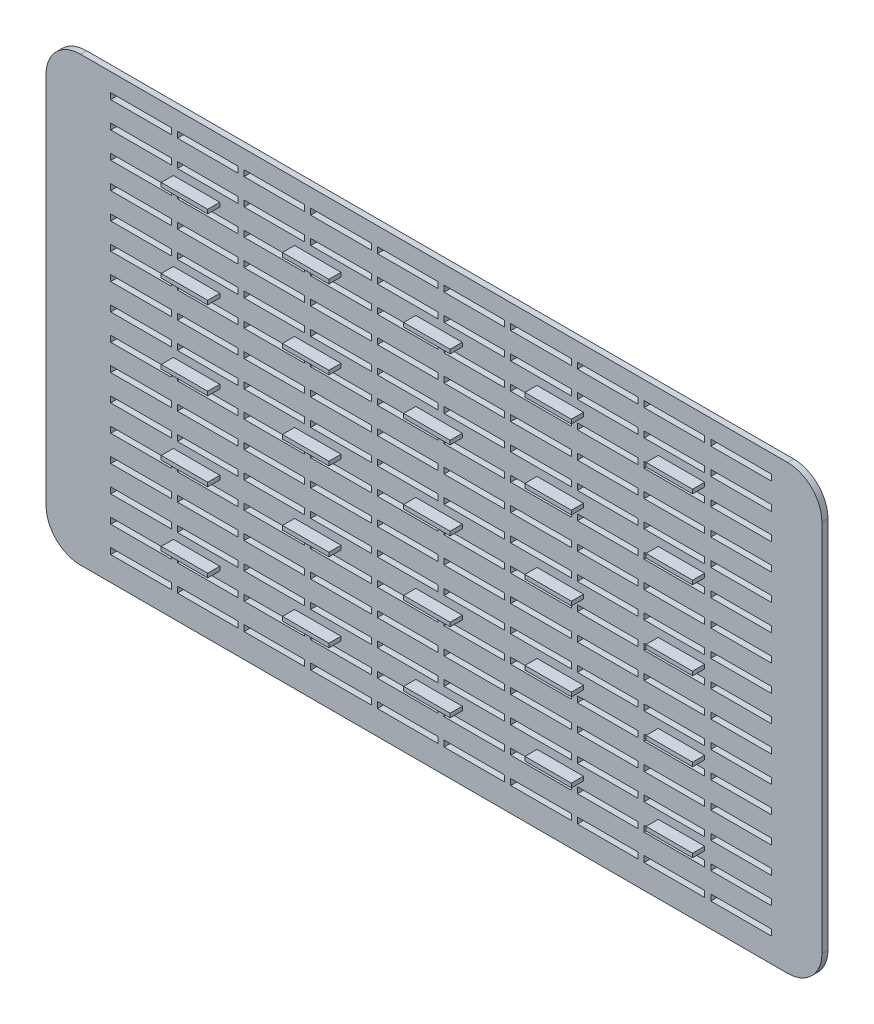
SolidWorks part; units mm, degrees
ref_plane "前视" through (0, 0, 0) normal (0, 0, 1) x (1, 0, 0)
ref_plane "上视" through (0, 0, 0) normal (0, 1, 0) x (1, 0, 0)
ref_plane "右视" through (0, 0, 0) normal (1, 0, 0) x (0, 0, -1)
sketch "草图1" plane through (0, 0, 0) normal (0, 0, 1) x (1, 0, 0)
  line L1 (-192, -109.5) -> (192, -109.5)
  line L2 (-192, -109.5) -> (-192, 109.5)
  line L3 (-192, 109.5) -> (192, 109.5)
  line L4 (192, -109.5) -> (192, 109.5)
  line L5 (-192, -109.5) -> (192, 109.5) construction
  line L6 (-192, 109.5) -> (192, -109.5) construction
  point P0 (0, 0)
  dimension "D1" = 384
  dimension "D2" = 219
extrude "凸台-拉伸1" add sketch "草图1" along normal blind 3
fillet "圆角1" radius 17 4 edges at (-192, -109.5, 1.5) (-192, 109.5, 1.5) (192, -109.5, 1.5) (192, 109.5, 1.5)
sketch "草图2" plane through (0, 0, 3) normal (0, 0, 1) x (1, 0, 0)
  line L0 (175, 109.5) -> (-175, 109.5) construction
  line L1 (-160, 100.5) -> (-130, 100.5)
  line L2 (-160, 100.5) -> (-160, 97.5)
  line L3 (-160, 97.5) -> (-130, 97.5)
  line L4 (-130, 100.5) -> (-130, 97.5)
  dimension "D1" = 30
  dimension "D2" = 3
  dimension "D3" = 160
  dimension "D4" = 9
extrude "切除-拉伸1" cut sketch "草图2" against normal blind 3
pattern_linear "阵列(线性)1" count 10 spacing 33 along (1, 0, 0) count 16 spacing 13 along (0, -1, 0) of "切除-拉伸1"
sketch "草图3" plane through (0, 0, 3) normal (0, 0, 1) x (1, 0, 0)
  line L0 (0, 0) -> (0, 105.2506) construction
  line L1 (-129, 80.5005) -> (-106, 80.5005)
  line L2 (-129, 80.5005) -> (-129, 78.5005)
  line L3 (-129, 78.5005) -> (-106, 78.5005)
  line L4 (-106, 80.5005) -> (-106, 78.5005)
  line L5 (0, 0) -> (-107.6391, 0) construction
  line L18 (-192, 92.5) -> (-192, -92.5) construction
  point P7 (-130, 80.5005)
  point P14 (-142, 65.1864)
  point P15 (-142, 26.6596)
  dimension "D1" = 2
  dimension "D3" = 23
  dimension "D4" = 63
extrude "凸台-拉伸2" add sketch "草图3" along normal blind 6
pattern_linear "阵列(线性)2" count 5 spacing 39 along (0, -1, 0) count 5 spacing 60 along (1, 0, 0) of "凸台-拉伸2"
